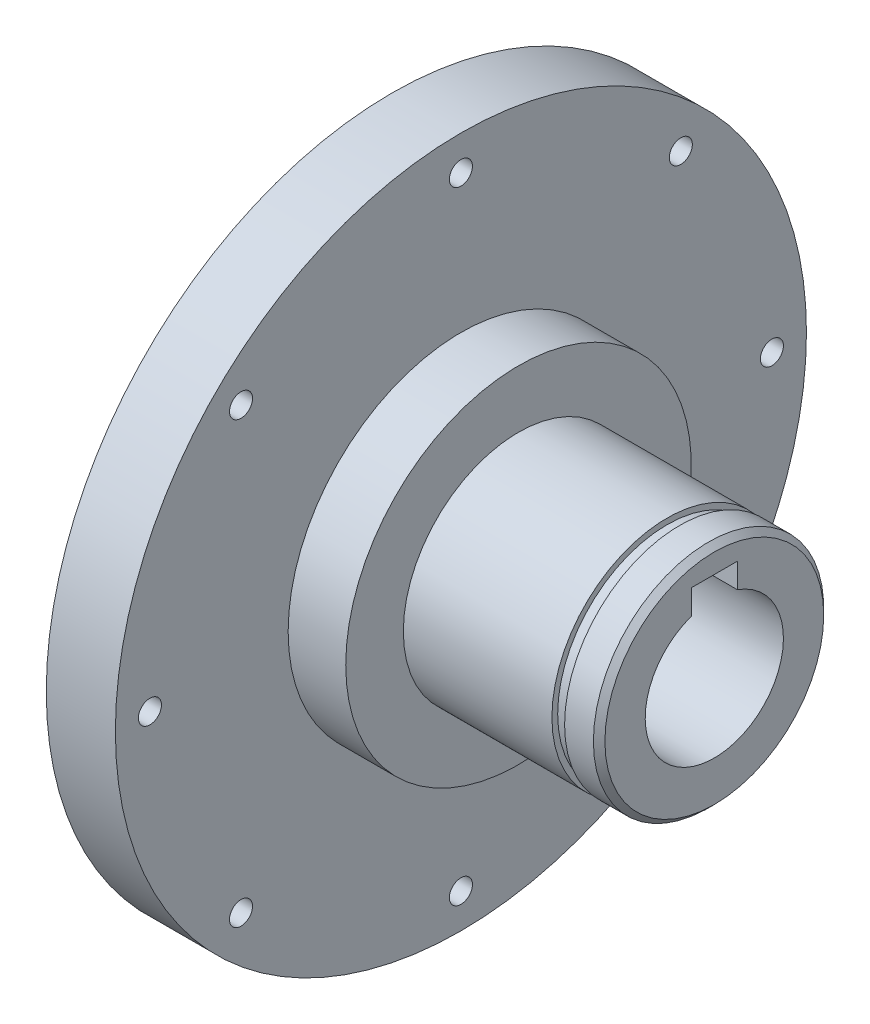
SolidWorks part; units mm, degrees
material "6061-T6 (SS)"
ref_plane "前视基准面" through (0, 0, 0) normal (0, 0, 1) x (1, 0, 0)
ref_plane "上视基准面" through (0, 0, 0) normal (0, 1, 0) x (1, 0, 0)
ref_plane "右视基准面" through (0, 0, 0) normal (1, 0, 0) x (0, 0, -1)
other "Configuration Table"
sketch "草图1" plane through (0, 0, 0) normal (0, 0, 1) x (1, 0, 0)
  line L0 (0, 0) -> (12, 0)
  dimension "D1" = 12
revolve "旋转-薄壁2" add sketch "草图1" angle 360 about L0 wall 60
sketch "草图2" plane through (0, 0, 0) normal (0, 0, 1) x (1, 0, 0)
  line L0 (12, 0) -> (22, 0)
  line L1 (12, -60) -> (12, 60) construction
  dimension "D1" = 10
revolve "旋转-薄壁4" add sketch "草图2" angle 360 about L0 wall 30
sketch "草图3" plane through (0, 0, 0) normal (0, 0, 1) x (1, 0, 0)
  line L0 (22, 0) -> (56, 0)
  line L1 (22, -30) -> (22, 30) construction
  dimension "D1" = 34
revolve "旋转-薄壁5" add sketch "草图3" angle 360 about L0 wall 20
sketch "草图4" plane through (0, 0, 0) normal (1, 0, 0) x (0, 0, -1)
  line L1 (-4, 15.6) -> (4, 15.6)
  line L2 (-4, 15.6) -> (-4, 11.3137)
  line L3 (4, 15.6) -> (4, 11.3137)
  arc A0 (-4, 11.3137) -> (4, 11.3137) centre (0, 0) ccw
  point P9 (0, 15.6)
  dimension "D1" = 24
  dimension "D3" = 8
extrude "切除-拉伸2" cut sketch "草图4" along normal through all
sketch "草图6" plane through (0, 0, 0) normal (1, 0, 0) x (0, 0, -1)
  circle A0 centre (0, 0) radius 19
  dimension "D1" = 38
extrude "切除-拉伸4" cut sketch "草图6" against normal blind 2.2 from offset 50 flip side to cut
sketch "草图7" plane through (0, 0, 0) normal (-1, 0, 0) x (0, 0, 1)
  circle A2 centre (0, 54) radius 2
  circle A3 centre (38.1838, 38.1838) radius 2
  circle A4 centre (54, 0) radius 2
  circle A5 centre (38.1838, -38.1838) radius 2
  circle A6 centre (0, -54) radius 2
  circle A7 centre (-38.1838, -38.1838) radius 2
  circle A8 centre (-54, 0) radius 2
  circle A9 centre (-38.1838, 38.1838) radius 2
  point P28 (0, 0)
  dimension "D2" = 4
  dimension "D3" = 8
extrude "切除-拉伸5" cut sketch "草图7" against normal through all
chamfer "倒角2" distance 1 angle 45 1 edges at (56, 0, 20)
